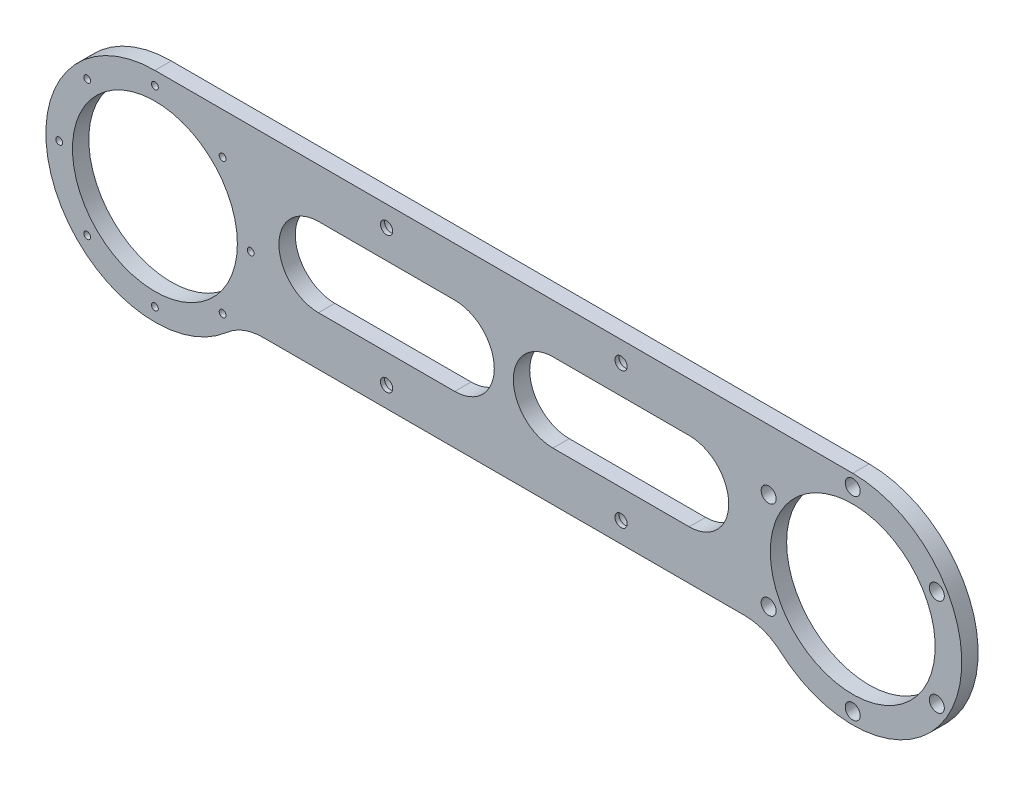
SolidWorks part; units mm, degrees
material "6061-T6 (SS)"
ref_plane "前视基准面" through (0, 0, 0) normal (0, 0, 1) x (1, 0, 0)
ref_plane "上视基准面" through (0, 0, 0) normal (0, 1, 0) x (1, 0, 0)
ref_plane "右视基准面" through (0, 0, 0) normal (1, 0, 0) x (0, 0, -1)
other "Configuration Table"
sketch "草图1" plane through (0, 0, 0) normal (0, 0, 1) x (1, 0, 0)
  line L1 (-128, 82.8866) -> (384, 82.8866)
  line L3 (-48.6275, -47.1134) -> (304.6275, -47.1134)
  line L4 (-8, 17.8866) -> (92, 17.8866) construction
  line L6 (-8, 46.8866) -> (92, 46.8866)
  line L10 (-8, -11.1134) -> (92, -11.1134)
  line L11 (164, 17.8866) -> (264, 17.8866) construction
  line L12 (164, 46.8866) -> (264, 46.8866)
  line L13 (164, -11.1134) -> (264, -11.1134)
  arc A0 (-128, 82.8866) -> (-75.085, -57.1134) centre (-128, 2.8866) ccw
  arc A1 (331.085, -57.1134) -> (384, 82.8866) centre (384, 2.8866) ccw
  arc A2 (-75.085, -57.1134) -> (-48.6275, -47.1134) centre (-48.6275, -87.1134) cw
  arc A3 (331.085, -57.1134) -> (304.6275, -47.1134) centre (304.6275, -87.1134) ccw
  circle A8 centre (-128, 2.8866) radius 60.5
  arc A10 (-8, 46.8866) -> (-8, -11.1134) centre (-8, 17.8866) ccw
  arc A11 (92, -11.1134) -> (92, 46.8866) centre (92, 17.8866) ccw
  arc A12 (164, 46.8866) -> (164, -11.1134) centre (164, 17.8866) ccw
  arc A13 (264, -11.1134) -> (264, 46.8866) centre (264, 17.8866) ccw
  point P4 (0, 0)
  point P9 (42, 17.8866)
  point P13 (128, -50)
  point P15 (42, 0)
  point P21 (214, 17.8866)
  point P22 (214, 0)
  dimension "D2" = 160
  dimension "D3" = 160
  dimension "D5" = 40
  dimension "D6" = 40
  dimension "D4" = 121
  dimension "D7" = 512
  dimension "D11" = 58
  dimension "D14" = 58
extrude "凸台-拉伸2" add sketch "草图1" along normal blind 12
sketch "草图3" plane through (0, 0, 0) normal (0, 0, 1) x (1, 0, 0)
  circle A0 centre (384, 2.8866) radius 60.5
  dimension "D2" = 121
extrude "切除-拉伸2" cut sketch "草图3" along normal blind 4
sketch "草图4" plane through (0, 0, 0) normal (0, 0, 1) x (1, 0, 0)
  line L0 (42, 46.8866) -> (42, 67.8866)
  line L1 (214, 67.8866) -> (214, 46.8866)
  line L2 (92, 46.8866) -> (-8, 46.8866) construction
  line L4 (42, -32.1134) -> (42, -11.1134)
  line L5 (-8, -11.1134) -> (92, -11.1134) construction
  line L6 (214, -32.1134) -> (214, -11.1134)
  line L7 (164, -11.1134) -> (264, -11.1134) construction
  point P11 (42, 17.8866)
  point P22 (214, 17.8866)
hole_wizard "M8 六角圆柱头螺钉的柱形沉头孔2" positions "草图9" profile "草图10" counterbore size "M8" standard "GB" end condition through all
sketch "草图9" plane through (0, 0, 0) normal (0, 0, -1) x (-1, 0, 0)
  point P0 (-214, 67.8866)
  point P3 (-214, -32.1134)
  point P6 (-42, 67.8866)
  point P9 (-42, -32.1134)
sketch "草图10" plane through (214, 67.8866, 0) normal (1, 0, 0) x (0, 1, 0)
  line L0 (0, 0) -> (0, 12)
  line L1 (0, 12) -> (4.5, 12)
  line L3 (4.5, 12) -> (4.5, 9)
  line L4 (4.5, 9) -> (7.5, 9)
  line L5 (7.5, 9) -> (7.5, 0)
  line L7 (7.5, 0) -> (0, 0)
  line L11 (0, -6.35) -> (0, 107.95) construction
  dimension "通孔孔直径" = 9
  dimension "通孔孔深度" = 12
  dimension "柱形沉头孔直径" = 15
  dimension "柱形沉头孔深度" = 9
sketch "草图11" plane through (0, 0, 0) normal (0, 0, 1) x (1, 0, 0)
  circle A0 centre (384, 2.8866) radius 18
  dimension "D2" = 36
extrude "切除-拉伸5" cut sketch "草图11" along normal through all
sketch "草图12" plane through (0, 0, 12) normal (0, 0, 1) x (1, 0, 0)
  circle A0 centre (-78.3257, 52.5608) radius 2.5
  circle A1 centre (-128, 73.1366) radius 2.5
  circle A2 centre (-57.75, 2.8866) radius 2.5
  circle A3 centre (-78.3257, -46.7877) radius 2.5
  circle A4 centre (-128, -67.3634) radius 2.5
  circle A5 centre (-177.6743, -46.7877) radius 2.5
  circle A6 centre (-198.25, 2.8866) radius 2.5
  circle A7 centre (-177.6743, 52.5608) radius 2.5
  point P13 (-128, 2.8866)
  point P28 (-128, 2.8866)
  dimension "D1" = 5
  dimension "D3" = 8
extrude "切除-拉伸6" cut sketch "草图12" against normal through all
sketch "草图13" plane through (0, 0, 4) normal (0, 0, -1) x (-1, 0, 0)
  circle A0 centre (-384, 2.8866) radius 60.5
extrude "切除-拉伸7" cut sketch "草图13" against normal through all
sketch "草图14" plane through (0, 0, 0) normal (0, 0, -1) x (-1, 0, 0)
  circle A0 centre (-384, 2.8866) radius 71.25 construction
  circle A1 centre (-384, 74.1366) radius 5.5
  circle A2 centre (-322.2957, 38.5116) radius 5.5
  circle A3 centre (-322.2957, -32.7384) radius 5.5
  circle A4 centre (-384, -68.3634) radius 5.5
  circle A5 centre (-445.7043, -32.7384) radius 5.5
  circle A6 centre (-445.7043, 38.5116) radius 5.5
  point P17 (-384, 2.8866)
  dimension "D1" = 142.5
  dimension "D2" = 11
  dimension "D3" = 6
extrude "切除-拉伸8" cut sketch "草图14" against normal through all
